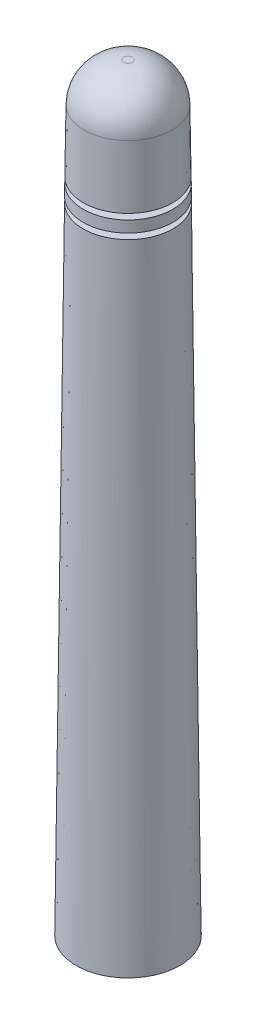
SolidWorks part; units mm, degrees
material "ABS"
ref_plane "前视基准面" through (0, 0, 0) normal (0, 0, 1) x (1, 0, 0)
ref_plane "上视基准面" through (0, 0, 0) normal (0, 1, 0) x (1, 0, 0)
ref_plane "右视基准面" through (0, 0, 0) normal (1, 0, 0) x (0, 0, -1)
sketch "草图1" plane through (0, 0, 0) normal (0, 0, 1) x (1, 0, 0)
  line L0 (-4.6, 0) -> (-4, 0)
  line L1 (-3.25, 58.3) -> (-3.25, 57.8)
  line L2 (-3.25, 56.8) -> (-3.25, 56.3)
  line L3 (-2.5755, 64.3) -> (-2.75, 10)
  line L6 (-0.3914, 67.3) -> (0, 67.3)
  line L7 (0, 67.3) -> (0, 65.3)
  line L8 (0, 0) -> (0, 72.8671) construction
  line L9 (-4, 4.3) -> (-4, 2.5)
  line L10 (-3.9691, 58.3) -> (-3.25, 58.3)
  line L11 (-3.5, 1) -> (-3.5, 2.5)
  line L12 (-3.9746, 57.8) -> (-3.25, 57.8)
  line L13 (-3.9857, 56.3) -> (-3.25, 56.3)
  line L15 (-4, 1) -> (-4, 0)
  line L16 (-3.9857, 56.8) -> (-3.25, 56.8)
  line L17 (-3.5, 4.3) -> (-3.5, 5.8)
  line L18 (0, 65.3) -> (-1.5755, 65.3)
  line L19 (-3.5, 1) -> (-4, 1)
  line L20 (-4, 7.3) -> (-3.5, 7.3)
  line L21 (-3.5, 7.3) -> (-3.5, 9.1)
  line L22 (-3.5, 9.1) -> (-4, 9.1)
  line L23 (-4, 7.3) -> (-4, 5.8)
  line L59 (-4, 10) -> (-4, 9.1)
  line L64 (-3.9857, 56.3) -> (-4.6, 0)
  line L65 (-3.9746, 57.8) -> (-3.9857, 56.8)
  line L66 (-3.8912, 63.8392) -> (-3.9691, 58.3)
  line L86 (-2.75, 10) -> (-4, 10)
  line L92 (-4, 5.8) -> (-3.5, 5.8)
  line L93 (-3.5, 4.3) -> (-4, 4.3)
  line L96 (-4, 2.5) -> (-3.5, 2.5)
  arc A0 (-2.5755, 64.3) -> (-1.5755, 65.3) centre (-1.5755, 64.3) cw
  arc A2 (-0.3914, 67.3) -> (-3.8912, 63.8392) centre (-0.3914, 63.8) ccw
  dimension "D2" = 3.5
  dimension "D19" = 1
  dimension "D1" = 0.5
  dimension "D3" = 67.3
  dimension "D4" = 2
  dimension "D5" = 9
  dimension "D6" = 1
  dimension "D7" = 0.5
  dimension "D8" = 5.5
  dimension "D9" = 6.5
  dimension "D10" = 9.2
  dimension "D11" = 1.5
  dimension "D12" = 0.5
  dimension "D13" = 1.8
  dimension "D14" = 1.5
  dimension "D15" = 1.5
  dimension "D16" = 1.8
  dimension "D17" = 8
  dimension "D18" = 7
revolve "旋转1" add sketch "草图1" angle 360 about L8
sketch "草图2" plane through (0, 0, 0) normal (0, -1, 0) x (1, 0, 0)
  line L0 (-4.8225, 0) -> (4.8225, 0) construction
  line L1 (0, 5.0407) -> (0, -5.0407) construction
  line L2 (-4.3742, 0.25) -> (-3.4, 0.25)
  line L3 (-4.3742, 0.25) -> (-4.3742, -0.25)
  line L4 (-4.3742, -0.25) -> (-3.4, -0.25)
  line L5 (-3.4, 0.25) -> (-3.4, -0.25)
  line L6 (3.4, 0.25) -> (3.4, -0.25)
  line L7 (4.3742, -0.25) -> (3.4, -0.25)
  line L8 (4.3742, 0.25) -> (4.3742, -0.25)
  line L9 (4.3742, 0.25) -> (3.4, 0.25)
  point P2 (0, 0)
  point P10 (0, 0)
  dimension "D1" = 0.5
  dimension "D2" = 6.8
extrude "凸台-拉伸1" add sketch "草图2" against normal up to surface (7.3 mm away) up to face at (0, 7.3, -3.5)
